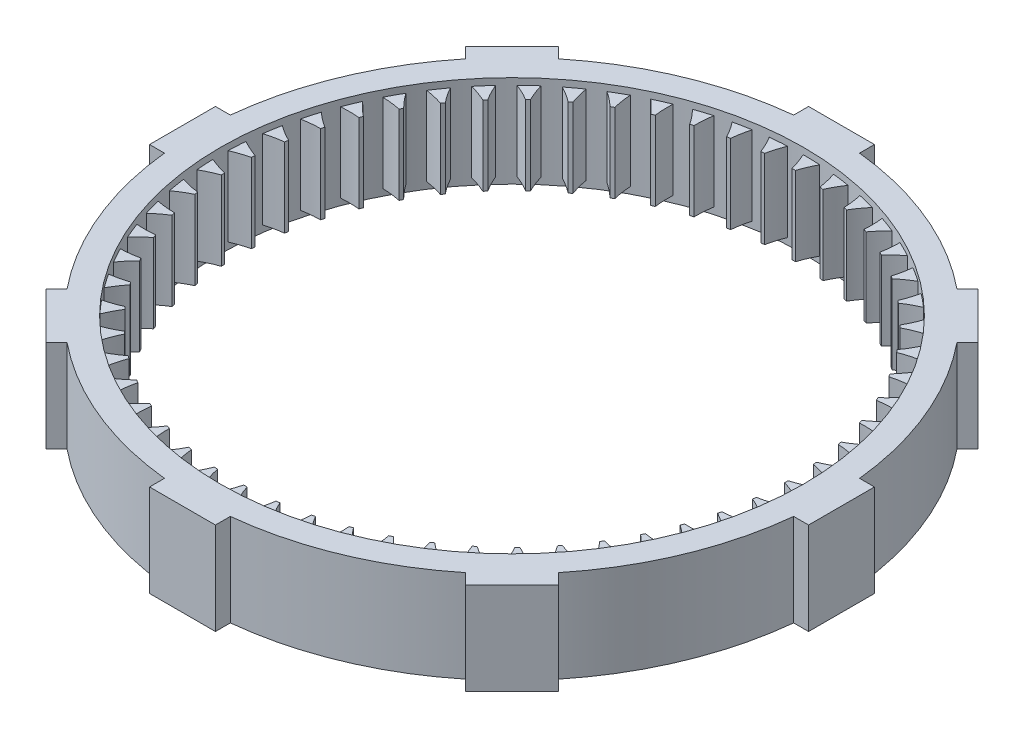
from build123d import *

# Parameters (mm, degrees)
SKETCH_1_3_R        = 44.25
BOSS_EXTRUDE1_DEPTH = 7
BOSS_EXTRUDE2_DEPTH = 6
CIRPATTERN1_COUNT   = 57


with BuildPart() as part:
    # Sketch 1_3 → Boss-Extrude1 (new, symmetric)
    with BuildSketch(Plane(origin=(0, 0, 0), x_dir=(1, 0, 0), z_dir=(0, 1, 0))):
        with BuildLine():
            Line((47.738873049, 5), (50, 5))
            Line((50, 5), (50, -5))
            Line((50, -5), (47.738873049, -5))
            ThreePointArc((47.738873049, -5), (44.346217561, -18.368804754), (37.292014765, -30.220946953))
            Line((37.292014765, -30.220946953), (38.890872965, -31.819805153))
            Line((38.890872965, -31.819805153), (31.819805153, -38.890872965))
            Line((31.819805153, -38.890872965), (30.220946953, -37.292014765))
            ThreePointArc((30.220946953, -37.292014765), (18.368804754, -44.346217561), (5, -47.738873049))
            Line((5, -47.738873049), (5, -50))
            Line((5, -50), (-5, -50))
            Line((-5, -50), (-5, -47.738873049))
            ThreePointArc((-5, -47.738873049), (-18.368804754, -44.346217561), (-30.220946953, -37.292014765))
            Line((-30.220946953, -37.292014765), (-31.819805153, -38.890872965))
            Line((-31.819805153, -38.890872965), (-38.890872965, -31.819805153))
            Line((-38.890872965, -31.819805153), (-37.292014765, -30.220946953))
            ThreePointArc((-37.292014765, -30.220946953), (-44.346217561, -18.368804754), (-47.738873049, -5))
            Line((-47.738873049, -5), (-50, -5))
            Line((-50, -5), (-50, 5))
            Line((-50, 5), (-47.738873049, 5))
            ThreePointArc((-47.738873049, 5), (-44.346217561, 18.368804754), (-37.292014765, 30.220946953))
            Line((-37.292014765, 30.220946953), (-38.890872965, 31.819805153))
            Line((-38.890872965, 31.819805153), (-31.819805153, 38.890872965))
            Line((-31.819805153, 38.890872965), (-30.220946953, 37.292014765))
            ThreePointArc((-30.220946953, 37.292014765), (-18.368804754, 44.346217561), (-5, 47.738873049))
            Line((-5, 47.738873049), (-5, 50))
            Line((-5, 50), (5, 50))
            Line((5, 50), (5, 47.738873049))
            ThreePointArc((5, 47.738873049), (18.368804754, 44.346217561), (30.220946953, 37.292014765))
            Line((30.220946953, 37.292014765), (31.819805153, 38.890872965))
            Line((31.819805153, 38.890872965), (38.890872965, 31.819805153))
            Line((38.890872965, 31.819805153), (37.292014765, 30.220946953))
            ThreePointArc((37.292014765, 30.220946953), (44.346217561, 18.368804754), (47.738873049, 5))
        make_face()
        with Locations(Location((0, 0, 0), (0, 0, 270))):
            Circle(SKETCH_1_3_R, mode=Mode.SUBTRACT)
    extrude(amount=BOSS_EXTRUDE1_DEPTH, both=True)

    # Sketch 1_3 2 → Boss-Extrude2 (add, symmetric)
    with BuildSketch(Plane(origin=(0, 0, 0), x_dir=(1, 0, 0), z_dir=(0, 1, 0))):
        with BuildLine():
            ThreePointArc((41.624151327, 0.265803086), (41.624787831, 0.13290222), (41.625, 0))
            ThreePointArc((41.625, 0), (41.624787831, -0.13290222), (41.624151327, -0.265803086))
            add(Edge.make_bspline(
                [(41.624151327, -0.265803086), (41.694869267, -0.285482539), (41.897877191, -0.343947574), (42.230936966, -0.448803587), (42.689963211, -0.611661941), (43.273555846, -0.844104445), (43.721288819, -1.043988352), (44.039124933, -1.196152418), (44.231141644, -1.291746457)],
                knots=[0.006786109, 0.006786109, 0.006786109, 0.006786109, 0.006786109, 0.008132613, 0.010661158, 0.013189703, 0.015718248, 0.019652819, 0.019652819, 0.019652819, 0.019652819, 0.019652819], degree=4))
            ThreePointArc((44.231141644, -1.291746457), (44.24528516, -0.645942054), (44.25, 0))
            ThreePointArc((44.25, 0), (44.24528516, 0.645942054), (44.231141644, 1.291746457))
            add(Edge.make_bspline(
                [(41.624151327, 0.265803086), (41.694869267, 0.285482539), (41.897877191, 0.343947574), (42.230936966, 0.448803587), (42.689963211, 0.611661941), (43.273555846, 0.844104445), (43.721288819, 1.043988352), (44.039124933, 1.196152418), (44.231141644, 1.291746457)],
                knots=[0.006786109, 0.006786109, 0.006786109, 0.006786109, 0.006786109, 0.008132613, 0.010661158, 0.013189703, 0.015718248, 0.019652819, 0.019652819, 0.019652819, 0.019652819, 0.019652819], degree=4))
        make_face()
    boss_extrude2 = extrude(amount=BOSS_EXTRUDE2_DEPTH, both=True)

    # CirPattern1: Boss-Extrude2 ×57 about axis
    cirpattern1_axis = Axis((0, 7, 0), (0, 1, 0))
    for i in range(1, CIRPATTERN1_COUNT):
        add(boss_extrude2.rotate(cirpattern1_axis, i * 360 / CIRPATTERN1_COUNT))


solid = part.part
